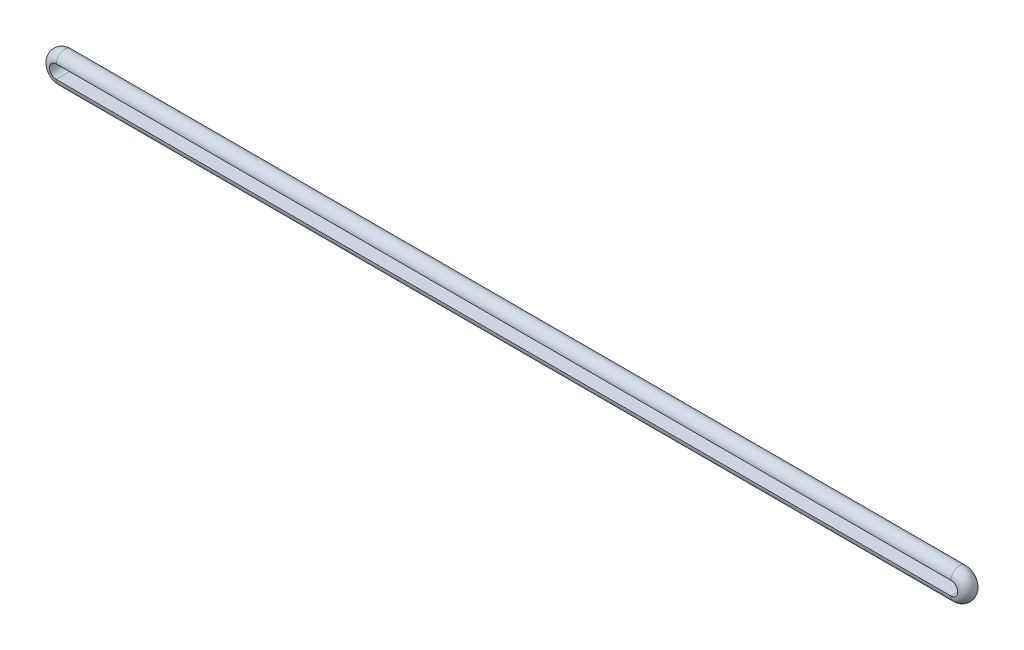
from build123d import *


with BuildPart() as part:
    # Sweep1: sweep along a path in Sketch1
    with BuildLine(Plane.XY) as sweep1_path:
        Line((0, 8), (1060, 8))
        ThreePointArc((1060, 8), (1068, 0), (1060, -8))
        Line((1060, -8), (0, -8))
        ThreePointArc((0, -8), (-8, 0), (0, 8))
    # Sketch2 → Sweep1 (sweep)
    with BuildSketch(Plane(origin=(0, 0, 0), x_dir=(0, 0, -1), z_dir=(1, 0, 0))):
        with BuildLine():
            Line((-10, 8), (10, 8))
            ThreePointArc((10, 8), (0, 18), (-10, 8))
        make_face()
    sweep(path=sweep1_path.line)


solid = part.part
